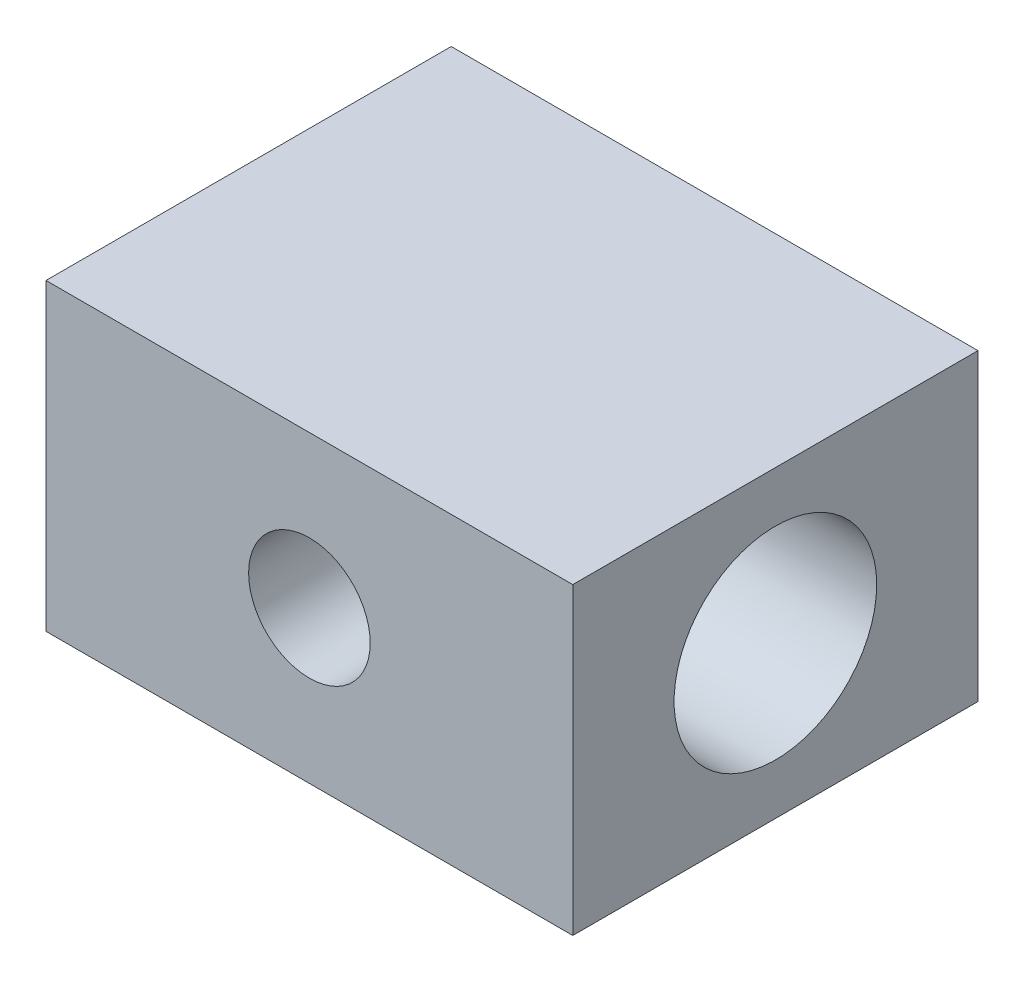
from build123d import *

# Parameters (mm, degrees)
SKETCH1_W           = 26
SKETCH1_H           = 15
SKETCH1_R           = 3
BOSS_EXTRUDE1_DEPTH = 20
SKETCH2_R           = 5
CUT_EXTRUDE1_DEPTH  = 34.648922717


with BuildPart() as part:
    # Sketch1 → Boss-Extrude1 (new body)
    with BuildSketch(Plane.XY):
        Rectangle(SKETCH1_W, SKETCH1_H)
        Circle(SKETCH1_R, mode=Mode.SUBTRACT)
    extrude(amount=BOSS_EXTRUDE1_DEPTH)

    # Sketch2 → Cut-Extrude1 (cut, through all)
    with BuildSketch(Plane(origin=(13, 0, 0), x_dir=(0, 0, -1), z_dir=(1, 0, 0))):
        with Locations((-10, 0)):
            Circle(SKETCH2_R)
    extrude(amount=-CUT_EXTRUDE1_DEPTH, mode=Mode.SUBTRACT)


solid = part.part
